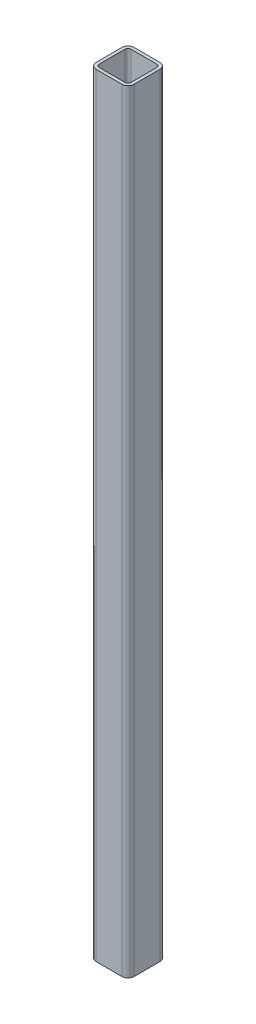
from build123d import *

# Parameters (mm, degrees)
GB_T_6728_2002_SQUARE_HOLLOW_SECTION_50_DEPTH = 1020


with BuildPart() as part:
    # Sketch1 → Gb／t 6728—2002 square hollow section 50×50×4(1) (new body)
    with BuildSketch(Plane(origin=(0, 0, 0), x_dir=(-1, 0, 0), z_dir=(0, 1, 0))):
        with BuildLine():
            Line((-17, -25), (17, -25))
            ThreePointArc((17, -25), (22.656854249, -22.656854249), (25, -17))
            Line((25, -17), (25, 17))
            ThreePointArc((25, 17), (22.656854249, 22.656854249), (17, 25))
            Line((17, 25), (-17, 25))
            ThreePointArc((-17, 25), (-22.656854249, 22.656854249), (-25, 17))
            Line((-25, 17), (-25, -17))
            ThreePointArc((-25, -17), (-22.656854249, -22.656854249), (-17, -25))
        make_face()
        with BuildLine():
            Line((-17, -21), (17, -21))
            ThreePointArc((17, -21), (19.828427125, -19.828427125), (21, -17))
            Line((21, -17), (21, 17))
            ThreePointArc((21, 17), (19.828427125, 19.828427125), (17, 21))
            Line((17, 21), (-17, 21))
            ThreePointArc((-17, 21), (-19.828427125, 19.828427125), (-21, 17))
            Line((-21, 17), (-21, -17))
            ThreePointArc((-21, -17), (-19.828427125, -19.828427125), (-17, -21))
        make_face(mode=Mode.SUBTRACT)
    extrude(amount=GB_T_6728_2002_SQUARE_HOLLOW_SECTION_50_DEPTH)


solid = part.part
